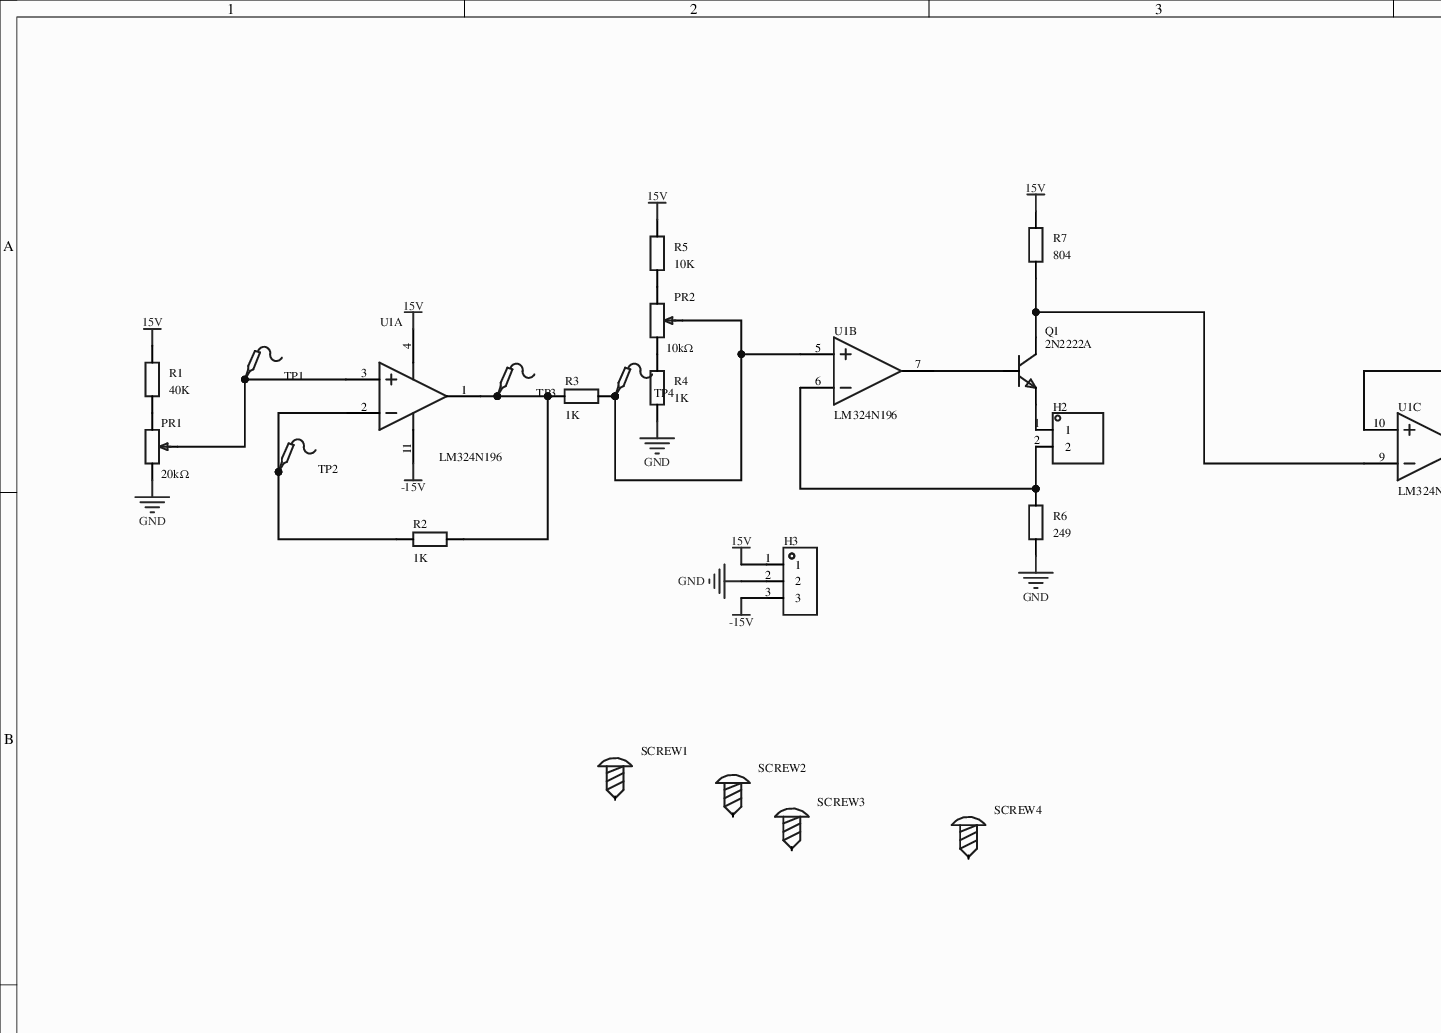
[diagram p0: MISC51286-3.schdoc, top left]
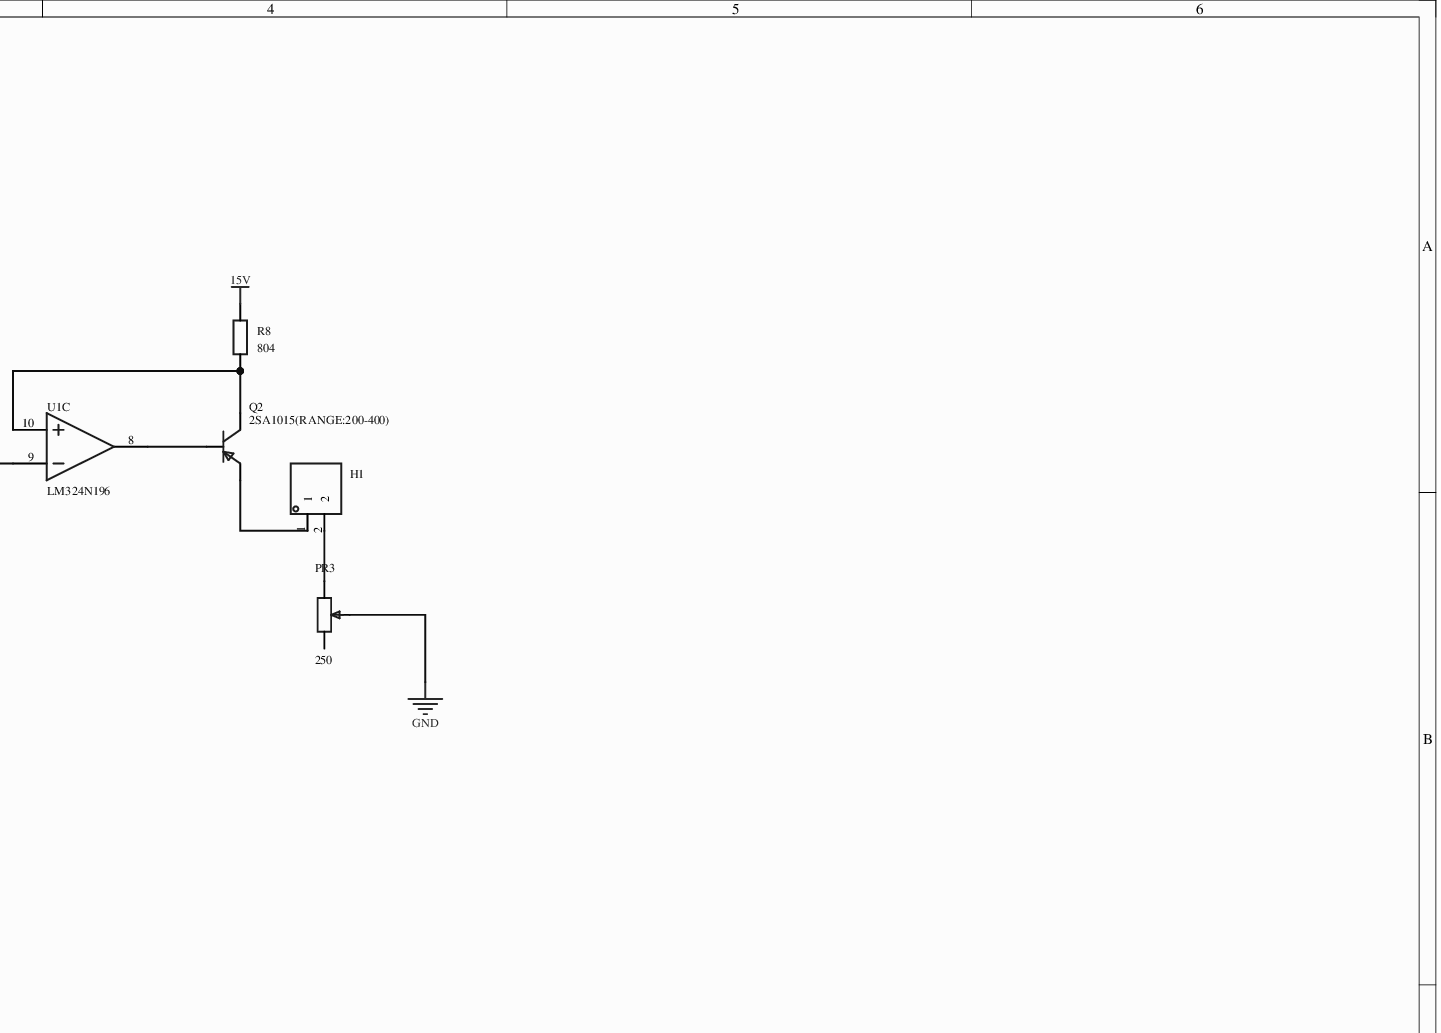
[diagram p1: MISC51286-3.schdoc, top right]
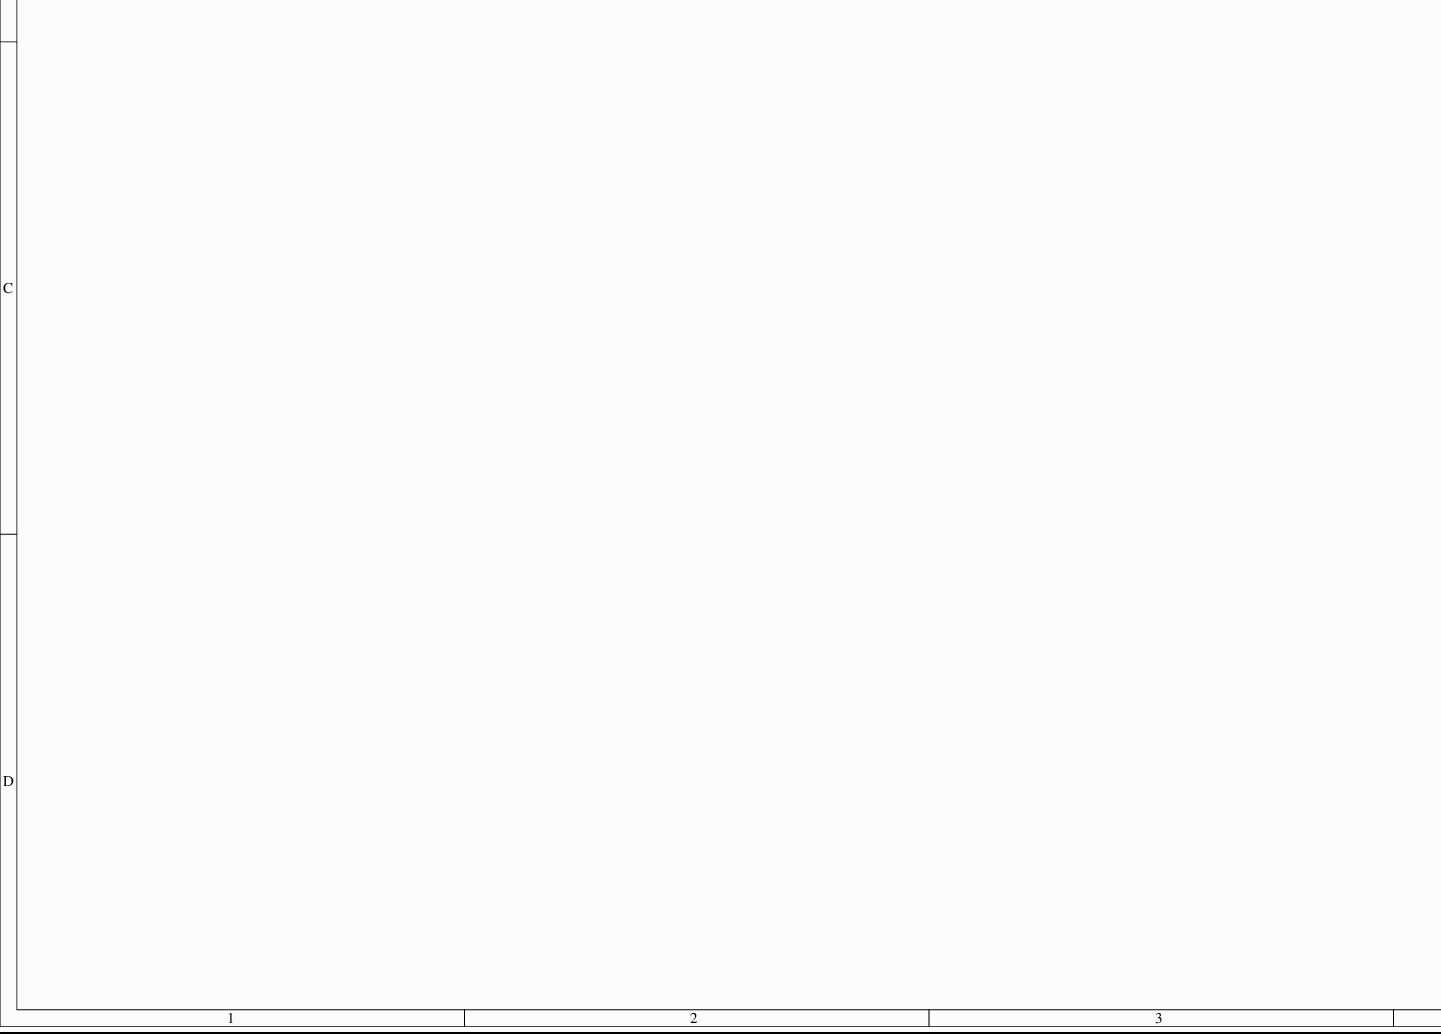
[diagram p2: MISC51286-3.schdoc, bottom left]
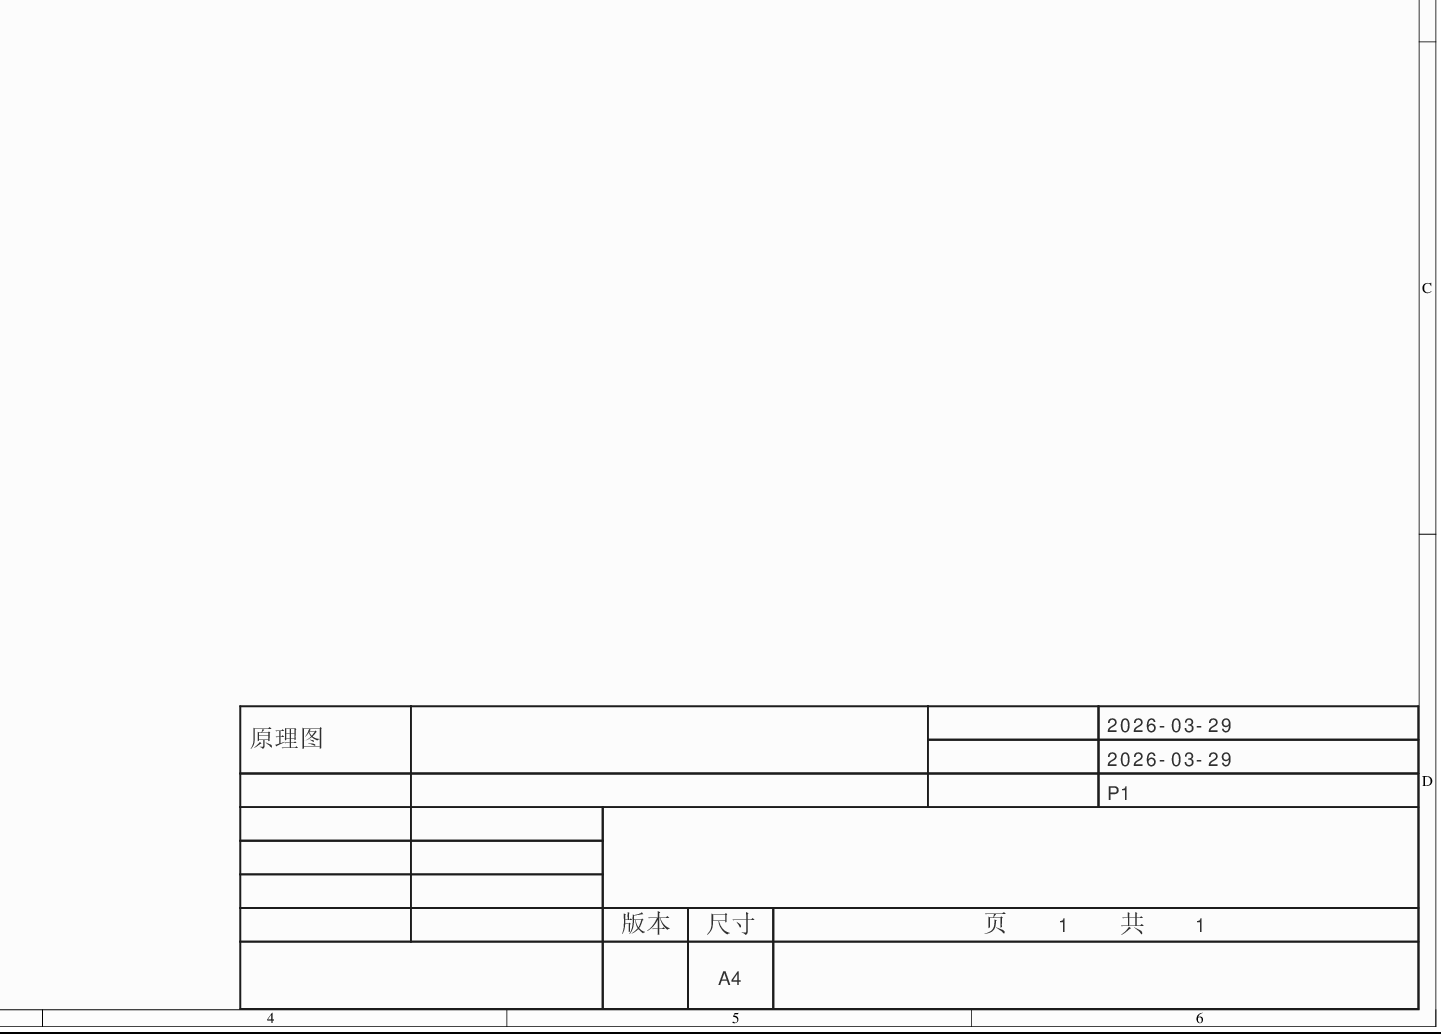
[diagram p3: MISC51286-3.schdoc, bottom right]
# Altium project MISC51286-2.PrjPcb
1 sheet, 25 parts. Net scope: global (net labels, ports and power ports of the same name join across sheets).
Board file: MISC51286.pcbdoc

## Sheet MISC51286-3.schdoc
size 420 x 297 mm; Version: V1.0; @Project Name: MISC51286; @Update Date: 2026-03-29; @Create Date: 2026-03-29; @Board Name: MISC51286; @Create Time: 13:06:10; @Page Count: 1; @Page No: 1; @Schematic Name: MISC51286; @Update Time: 13:06:10; Size: A4

### Parts
H1  (no value)  [HDR-TH_2P-P2.54-V-M-1]
H2  (no value)  [HDR-TH_2P-P2.54-V-M-1]
H3  (no value)  [HDR-TH_3P-P2.54-V-M]
PR1  20kΩ  [R_3296]
PR2  10kΩ  [R_3296]
PR3  250  [R_3296]
Q1  2N2222A  [TO-92-3_L5.1-W4.1-P1.27-L-1]
Q2  2SA1015(RANGE:200-400)  [TO-92-3_L4.9-W3.7-P1.27-L]
R1  40K  [R0805]
R2  1K  [R0805]
R3  1K  [R0805]
R4  1K  [R0805]
R5  10K  [R0805]
R6  249  [R0805]
R7  804  [R0805]
R8  804  [R0805]
SCREW1  (no value)  [M2螺丝]
SCREW2  (no value)  [M2螺丝]
SCREW3  (no value)  [M2螺丝]
SCREW4  (no value)  [M2螺丝]
TP1  (no value)  [Test-Point-0.5mm]
TP2  (no value)  [Test-Point-0.5mm]
TP3  (no value)  [Test-Point-0.5mm]
TP4  (no value)  [Test-Point-0.5mm]
U1  LM324N196  [PDIP-14_L19.3-W6.5-P2.54-LS7.6-BL]  (parts A,B,C of 4)

### Nets
15V: H3.1 R1.2 R5.1 R7.1 R8.1 U1.4(V-)
-15V: H3.3 U1.11(V+)
GND: H3.2 PR1.1 PR3.2 R4.2 R6.2
NetH1_1: H1.1 Q2.1(E)
NetH1_2: H1.2 PR3.3
NetH2_1: H2.1 Q1.1(E)
NetH2_2: H2.2 R6.1 U1.6(IN2-)
NetPR1_2: PR1.2 TP1.1 U1.3(IN1+)
NetPR1_3: PR1.3 R1.1
NetPR2_1: PR2.1 R4.1
NetPR2_2: PR2.2 R3.1 TP4.1 U1.5(IN2+)
NetPR2_3: PR2.3 R5.2
NetQ1_2: Q1.2(B) U1.7(OUT2)
NetQ1_3: Q1.3(C) R7.2 U1.9(IN3-)
NetQ2_2: Q2.2(C) R8.2 U1.10(IN3+)
NetQ2_3: Q2.3(B) U1.8(OUT3)
NetR2_1: R2.1 R3.2 TP3.1 U1.1(OUT1)
NetR2_2: R2.2 TP2.1 U1.2(IN1-)

Not connected (* = marked no-connect by the designer): PR3 1; SCREW1 1; SCREW2 1; SCREW3 1; SCREW4 1

### Notes on the sheet
- 2026-03-29
- 原理图
- P1
- 版本
- 尺寸
- A4
- 页    1    共    1

### Library data of the parts
H1 H2 = HDR-M_2.54_1x2P: Symbol: 210S-1*2P L=11.6MMGold-plated black; ConvertToPcb: yes; ModelId: 79b2e9f2d70a4d68a1b7098f27c6d4c50819f05c4eef4c71ace90d822a990e87; ModelName: HDR-M-2.54_1x2; ModelTransform: 200,100,0,0,0,0,0,0,-118.11; Device: HDR-M_2.54_1x2P; AddInBom: yes; SupplierPart: C124375; Supplier Footprint: 插件; FootprintName: HDR-TH_2P-P2.54-V-M-1
H3 = HDR-M_2.54_1x3P: AddInBom: yes; ModelId: bb473b6d38ff42a99216a4fcdbdcc4cb0819f05c4eef4c71ace90d822a990e87; ModelName: HDR-TH_3P-P2.54-M-LI-1X3P; ModelTransform: 300.03877,100,0,0,0,0,0,0,-118.11; Symbol: HDR-M_2.54_1x3P; Device: HDR-M_2.54_1x3P; ConvertToPcb: yes; FootprintName: HDR-TH_3P-P2.54-V-M; SupplierPart: C2937625; Supplier Footprint: 插件
PR1-PR3 = R_3296: ConvertToPcb: yes; ModelId: b182808559bb43bda9e7de64b64134cb0819f05c4eef4c71ace90d822a990e87; ModelName: 3296W; ModelTransform: 373.98,188.96,590.49,180,0,0,0,0,-140; Symbol: R_3296; Device: R_3296; AddInBom: yes; Supplier Footprint: 直插; FootprintName: R_3296
  PR1: Value: 20kΩ
  PR2: Value: 10kΩ
  PR3: Value: 250
Q1 = 2N2222A_C50229645: 晶体管类型：NPN。                 集电极电流ICM:800MA                    集电极-基极击穿电压BVCBO:60V      集电极-发射极击穿电压BVCEO:30V      直流电流增益HFE:100-200; Manufacturer: DDF(鼎德丰); AddInBom: yes; ModelId: 3974197e164648709a3727be714795da0819f05c4eef4c71ace90d822a990e87; ModelTransform: 200.42283,161.417,0,0,0,0,0,9.842,-196.85; Symbol: 2N2222A_C50229645; Device: 2N2222A_C50229645; LCSC Part Name: 2N2222A; SupplierPart: C50229645; ManufacturerPart: 2N2222A; Supplier Footprint: TO-92; JLCPCB Part Class: Extended Part; Datasheet: https://item.szlcsc.com/datasheet/2N2222A/52814798.html; Supplier: LCSC; ConvertToPcb: yes; FootprintName: TO-92-3_L5.1-W4.1-P1.27-L-1; ModelName: TO-92-3_L5.1-W4.1-P1.27-L-1
Q2 = 2SA1015(RANGE:200-400): 晶体管类型:PNP;集电极电流(Ic):150mA;集射极击穿电压(Vceo):50V;耗散功率(Pd):400mW;直流电流增益(hFE):200@2mA,6V;; Manufacturer: CJ(江苏长电/长晶); Symbol: 2SA1015_C168617; AddInBom: yes; ModelId: aafe8e06f2154e7c93506efd0d6632dd0819f05c4eef4c71ace90d822a990e87; ModelTransform: 176.28752,144.88554,0,180,0,0,0,20.669,-196.85; type: PNP; Current - Collector(Ic): 150mA; Collector - Emitter Voltage VCEO: 50V; Pd - Power Dissipation: 400mW; Transition frequency(fT): 80MHz; Current - Collector Cutoff: 100nA; Vce Saturation(VCE(sat)): 300mV@100mA,10mA; Emitter-Base Voltage(Vebo): 5V; Number: 1个PNP; Device: 2SA1015(RANGE:200-400); LCSC Part Name: GR档(200~400) PNP 电流:150mA 电压:50V; SupplierPart: C168617; ManufacturerPart: 2SA1015(RANGE:200-400); Supplier Footprint: TO-92; JLCPCB Part Class: Extended Part; Datasheet: https://item.szlcsc.com/datasheet/2SA1015(RANGE%253A200-400)/180000.html; Supplier: LCSC; ConvertToPcb: yes; FootprintName: TO-92-3_L4.9-W3.7-P1.27-L; ModelName: TO-92-3_L4.9-W3.7-P1.27-L; DC Current Gain: 200@2mA,6V; Operating Temperature: -55℃~+150℃
R1-R8 = Res_0805: Symbol: 电阻; ConvertToPcb: yes; ModelId: 37a81e68749a4138bd2dfa6897b24b850819f05c4eef4c71ace90d822a990e87; ModelName: R0805_L2.0-W1.3-H0.6; ModelTransform: 78.74,51.181,0,0,0,0,0,-0.0005,0; Device: Res_0805; AddInBom: yes; Supplier Footprint: 0805; FootprintName: R0805
  R1: Value: 40K
  R2-R4: Value: 1K
  R5: Value: 10K
  R6: Value: 249
  R7 R8: Value: 804
SCREW1-SCREW4 = M2螺丝: Symbol: 螺丝孔; ConvertToPcb: yes; Device: M2螺丝; AddInBom: yes; Supplier Footprint: 插件; FootprintName: M2螺丝
TP1-TP4 = Test-Point: Test Point 测试点; AddInBom: yes; Symbol: Test-Point; Device: Test-Point; ConvertToPcb: yes; FootprintName: Test-Point-0.5mm
U1 = LM324N196: 放大器数:4;轨到轨:-;增益带宽积(GBW):-;输入失调电压(Vos):2mV;压摆率(SR):400V/ms;输入偏置电流(Ib):250nA;; Manufacturer: GMIC(绿微); Relevance: []; AddInBom: yes; ModelId: 7604059b31ae49f98a0332a7cce2343e0819f05c4eef4c71ace90d822a990e87; ModelTransform: 759.15391,311.417,0,0,0,0,0,0,-129.921; Number of Channels: 4; Maximum Power Supply Range (Vdd-Vss): 24V; Vos - Input Offset Voltage: 2mV; Input Offset Voltage Drift(Vos TC): 7uV/℃; Ib - Input Bias Current: 250nA; Input Offset Current(Ios): 5nA; Common Mode Rejection Ratio(CMRR): 80dB; Quiescent Current: 600uA; Output Current: 40mA; Single supply: 3V~24V; Dual Supply: -12V~-1.5V；1.5V~12V; Symbol: LM324N196; Device: LM324N196; LCSC Part Name: 高性能四独立运算放大器; SupplierPart: C51026325; ManufacturerPart: LM324N196; Supplier Footprint: DIP-14; JLCPCB Part Class: Extended Part; Datasheet: https://item.szlcsc.com/datasheet/LM324N196/53673003.html; Supplier: LCSC; ConvertToPcb: yes; FootprintName: PDIP-14_L19.3-W6.5-P2.54-LS7.6-BL; ModelName: PDIP-14_L19.3-W6.5-P2.54-LS7.6-BL; Rail to Rail: -; Gain Bandwidth Product: -; Slew Rate: 400V/ms; Input offset current drift(Ios TC): -; Operating Temperature: 0℃~+70℃